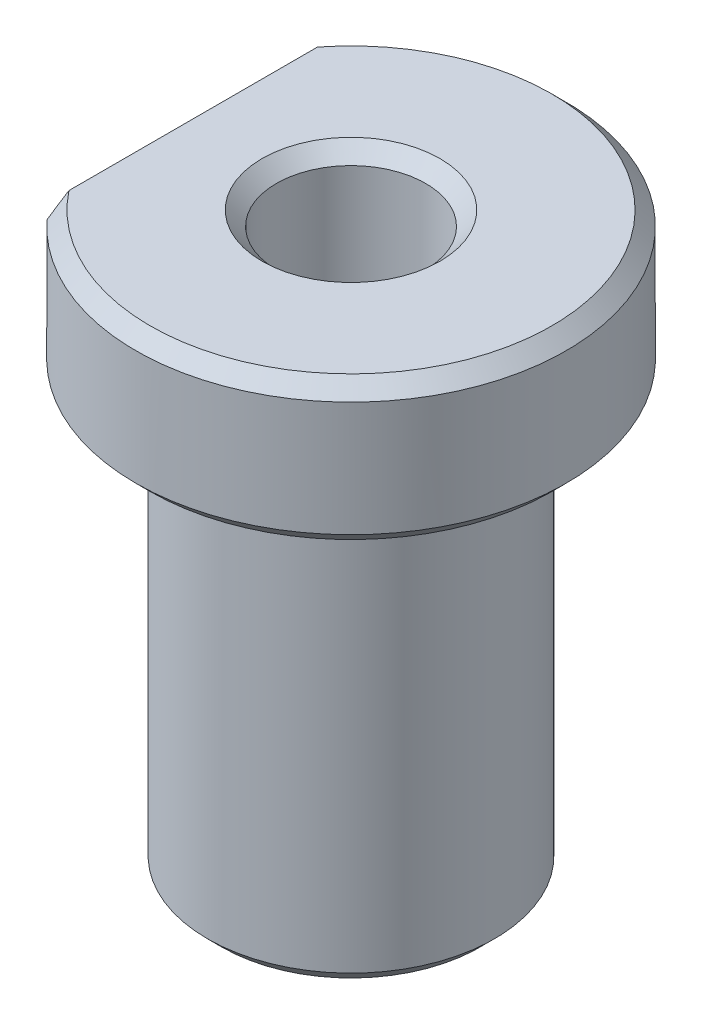
from build123d import *

# Parameters (mm, degrees)
SKETCH1_R           = 5
SKETCH1_R_2         = 2.6
BOSS_EXTRUDE1_DEPTH = 15
SKETCH2_R           = 7.5
SKETCH2_R_2         = 2.6
BOSS_EXTRUDE2_DEPTH = 5
CHAMFER1_SIZE       = 0.5
SKETCH3_W           = 5
SKETCH3_H           = 5
CUT_EXTRUDE1_DEPTH  = 25


with BuildPart() as part:
    # Sketch1 → Boss-Extrude1 (new body)
    with BuildSketch(Plane(origin=(0, 0, 0), x_dir=(1, 0, 0), z_dir=(0, 1, 0))):
        with Locations(Location((0, 0, 0), (0, 0, 270))):
            Circle(SKETCH1_R)
        with Locations(Location((0, 0, 0), (0, 0, 270))):
            Circle(SKETCH1_R_2, mode=Mode.SUBTRACT)
    extrude(amount=BOSS_EXTRUDE1_DEPTH)

    # Sketch2 → Boss-Extrude2 (add)
    with BuildSketch(Plane(origin=(0, 15, 0), x_dir=(1, 0, 0), z_dir=(0, 1, 0))):
        with Locations(Location((0, 0, 0), (0, 0, 270))):
            Circle(SKETCH2_R)
        with Locations(Location((0, 0, 0), (0, 0, 270))):
            Circle(SKETCH2_R_2, mode=Mode.SUBTRACT)
    extrude(amount=BOSS_EXTRUDE2_DEPTH)

    # Chamfer1
    chamfer1_edges = [part.edges().sort_by_distance(p)[0] for p in [
        (0, 20, -7.5),
        (0, 15, -7.5),
        (0, 20, -2.6),
        (0, 0, -5),
    ]]
    chamfer(chamfer1_edges, length=CHAMFER1_SIZE)

    # Sketch3 → Cut-Extrude1 (cut, symmetric)
    with BuildSketch(Plane.XY):
        with Locations((-8, 20.5)):
            Rectangle(SKETCH3_W, SKETCH3_H)
    extrude(amount=CUT_EXTRUDE1_DEPTH, both=True, mode=Mode.SUBTRACT)


solid = part.part
